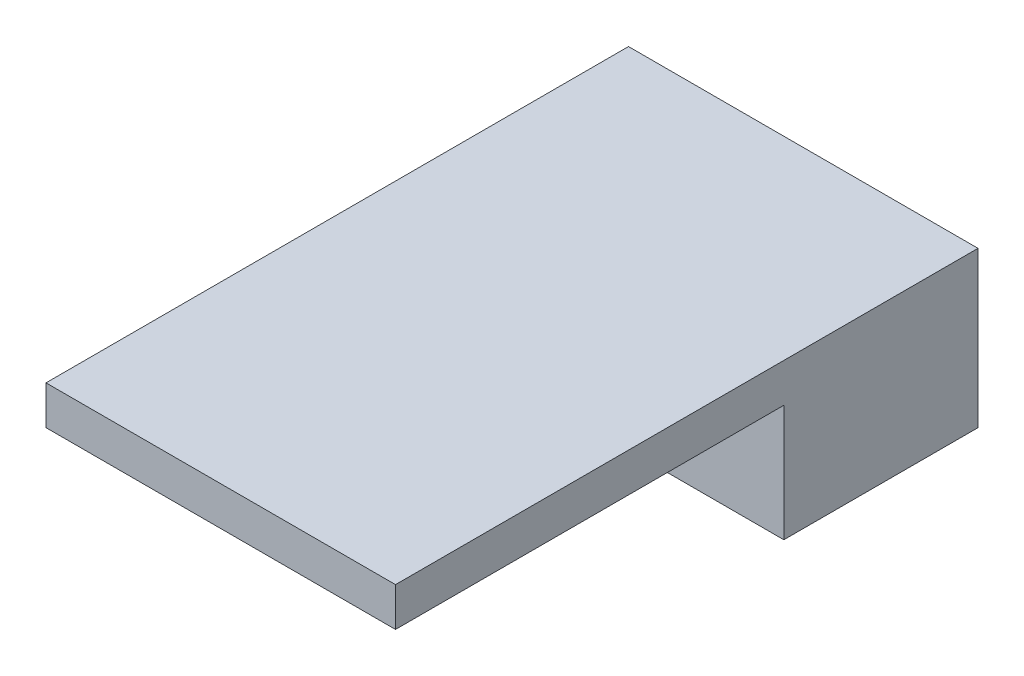
from build123d import *

# Parameters (mm, degrees)
SKETCH_1_W      = 18
SKETCH_1_H      = 8
EXTRUDE_1_DEPTH = 10
SKETCH_2_W      = 18
SKETCH_2_H      = 2
EXTRUDE_2_DEPTH = 20


with BuildPart() as part:
    # 草图1 → 凸台-拉伸1 (new body)
    with BuildSketch(Plane.XY):
        Rectangle(SKETCH_1_W, SKETCH_1_H)
    extrude(amount=EXTRUDE_1_DEPTH)

    # 草图2 → 凸台-拉伸2 (add)
    with BuildSketch(Plane.XY.offset(10)):
        with Locations((0, 3)):
            Rectangle(SKETCH_2_W, SKETCH_2_H)
    extrude(amount=EXTRUDE_2_DEPTH)

    # 草图3 → M3 螺纹孔1 (revolve, cut)
    with BuildSketch(Plane.YZ.offset(5)):
        Polygon((0, 0), (0, 7.251075774), (1.25, 6.5), (1.25, 0.275), (1.525, 0), align=None)
    hole_wizard_m3_1 = revolve(axis=Axis((5, 0, -6.35), (0, 0, 1)), mode=Mode.SUBTRACT)

    # 镜向1: M3 螺纹孔1 across plane
    add(hole_wizard_m3_1.mirror(Plane(origin=(0, 0, 0), x_dir=(0, 0, 1), z_dir=(1, 0, 0))), mode=Mode.SUBTRACT)


solid = part.part
